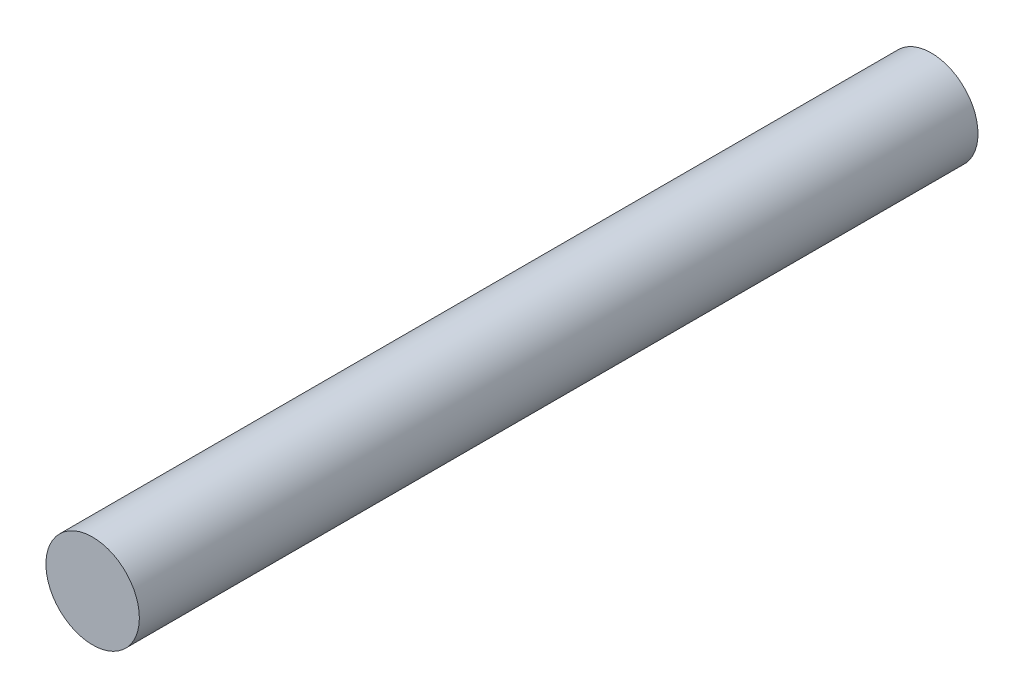
SolidWorks part; units mm, degrees
ref_plane "Front Plane" through (0, 0, 0) normal (0, 0, 1) x (1, 0, 0)
ref_plane "Top Plane" through (0, 0, 0) normal (0, 1, 0) x (1, 0, 0)
ref_plane "Right Plane" through (0, 0, 0) normal (1, 0, 0) x (0, 0, -1)
sketch "Sketch1" plane through (0, 0, 0) normal (0, 0, 1) x (1, 0, 0)
  circle A0 centre (8, -61.7532) radius 3.9
  dimension "D1" = 7.8
extrude "Boss-Extrude1" add sketch "Sketch1" along normal blind 70
